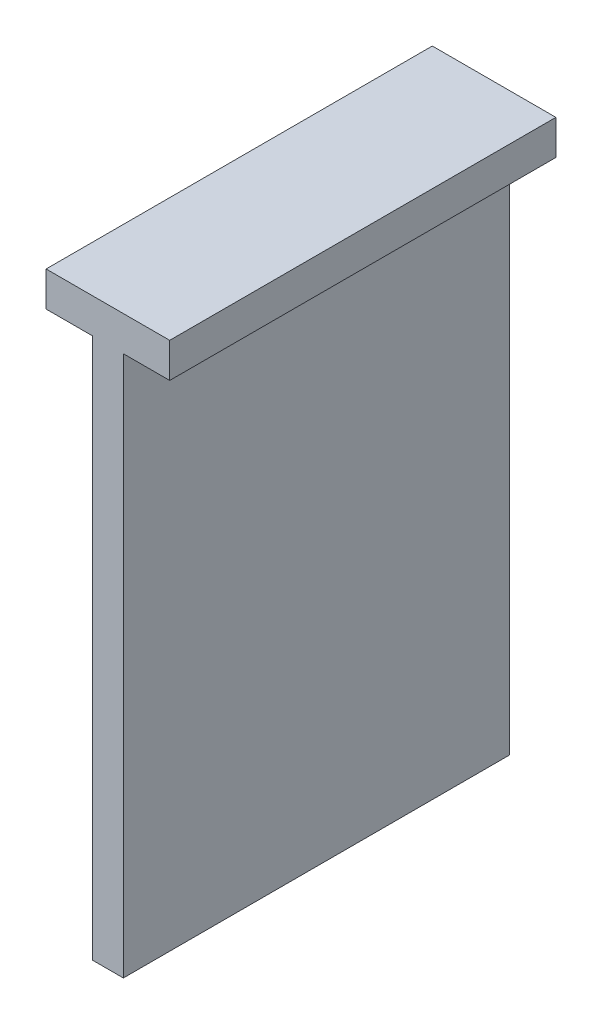
from build123d import *

# Parameters (mm, degrees)
EXTRUDE_1_DEPTH = 100


with BuildPart() as part:
    # 草图1 → 凸台-拉伸1 (new body)
    with BuildSketch(Plane.XY):
        Polygon((-32.039764657, -6.511895803), (-32.039764657, -120.09527648), (-32.039764657, -146.511895803), (-24.039764657, -146.511895803), (-24.039764657, -120.09527648), (-24.039764657, -6.511895803), (-12.039764657, -6.511895803), (-12.039764657, 2.488104197), (-44.039764657, 2.488104197), (-44.039764657, -6.511895803), align=None)
    extrude(amount=EXTRUDE_1_DEPTH)


solid = part.part
